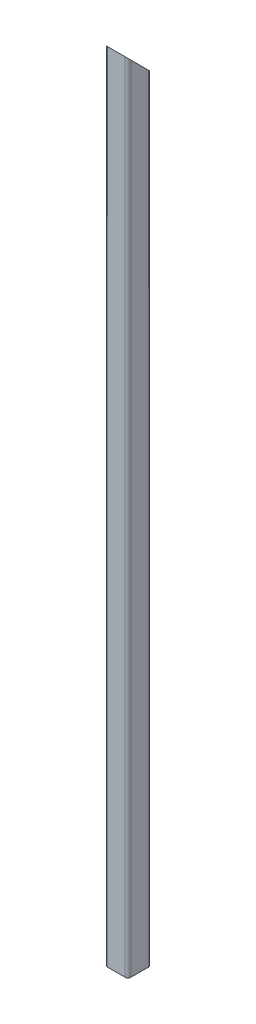
SolidWorks part; units mm, degrees
ref_plane "Front" through (0, 0, 0) normal (0, 0, 1) x (1, 0, 0)
ref_plane "Top" through (0, 0, 0) normal (0, 1, 0) x (1, 0, 0)
ref_plane "Right" through (0, 0, 0) normal (1, 0, 0) x (0, 0, -1)
sketch "草图1" plane through (0, 0, 0) normal (0, 1, 0) x (1, 0, 0)
  line L0 (-19, -7.2781) -> (19, -7.2781)
  line L1 (-19, -12.2781) -> (19, -12.2781)
  line L2 (-25, -6.2781) -> (-25, 31.7219)
  line L3 (-19, 37.7219) -> (19, 37.7219)
  line L4 (25, -6.2781) -> (25, 31.7219)
  line L5 (20, -6.2781) -> (20, 31.7219)
  line L6 (-19, 32.7219) -> (19, 32.7219)
  line L11 (-20, -6.2781) -> (-20, 31.7219)
  arc A0 (-19, -12.2781) -> (-25, -6.2781) centre (-19, -6.2781) cw
  arc A1 (19, -12.2781) -> (25, -6.2781) centre (19, -6.2781) ccw
  arc A2 (19, 37.7219) -> (25, 31.7219) centre (19, 31.7219) cw
  arc A3 (-25, 31.7219) -> (-19, 37.7219) centre (-19, 31.7219) cw
  arc A4 (19, -7.2781) -> (20, -6.2781) centre (19, -6.2781) ccw
  arc A5 (19, 32.7219) -> (20, 31.7219) centre (19, 31.7219) cw
  arc A6 (-20, 31.7219) -> (-19, 32.7219) centre (-19, 31.7219) cw
  arc A7 (-19, -7.2781) -> (-20, -6.2781) centre (-19, -6.2781) cw
  point P9 (25, -12.2781)
  point P12 (25, 37.7219)
  point P15 (-25, 37.7219)
  dimension "D3" = 6
  dimension "D1" = 50
  dimension "D2" = 50
  dimension "D4" = 5
extrude "凸台-拉伸1" add sketch "草图1" along normal blind 1775
sketch "草图2" plane through (25, 0, 0) normal (1, 0, 0) x (0, 0, -1)
  line L0 (-12.2781, 1775) -> (37.7219, 1775)
  line L1 (37.7219, 1775) -> (37.7219, 1725)
  line L2 (37.7219, 1775) -> (37.7219, 0) construction
  line L3 (37.7219, 1725) -> (-12.2781, 1775)
  dimension "D1" = 45
extrude "切除-拉伸1" cut sketch "草图2" against normal through all
sketch "草图3" plane through (0, 0, 0) normal (0, -1, 0) x (1, 0, 0)
  line L4 (-25, 6.2781) -> (-25, -31.7219)
  line L5 (-19, -37.7219) -> (19, -37.7219)
  line L6 (25, -31.7219) -> (25, 6.2781)
  line L7 (19, 12.2781) -> (-19, 12.2781)
  line L8 (-25, 6.2781) -> (-25, -31.7219)
  line L9 (-19, -37.7219) -> (19, -37.7219)
  line L10 (25, -31.7219) -> (25, 6.2781)
  line L11 (19, 12.2781) -> (-19, 12.2781)
  arc A4 (-19, 12.2781) -> (-25, 6.2781) centre (-19, 6.2781) ccw
  arc A5 (-25, -31.7219) -> (-19, -37.7219) centre (-19, -31.7219) ccw
  arc A6 (19, -37.7219) -> (25, -31.7219) centre (19, -31.7219) ccw
  arc A7 (25, 6.2781) -> (19, 12.2781) centre (19, 6.2781) ccw
  arc A8 (-19, 12.2781) -> (-25, 6.2781) centre (-19, 6.2781) ccw
  arc A9 (-25, -31.7219) -> (-19, -37.7219) centre (-19, -31.7219) ccw
  arc A10 (19, -37.7219) -> (25, -31.7219) centre (19, -31.7219) ccw
  arc A11 (25, 6.2781) -> (19, 12.2781) centre (19, 6.2781) ccw
  dimension "D1" = 0
extrude "凸台-拉伸2" add sketch "草图3" against normal blind 5
sketch "草图4" plane through (25, 0, 0) normal (1, 0, 0) x (0, 0, -1)
  line L0 (-6.2781, 0) -> (31.7219, 0) construction
  line L1 (-341.2655, 50) -> (254.9238, 50)
  line L2 (-341.2655, 50) -> (-341.2655, -272.9358)
  line L3 (-341.2655, -272.9358) -> (254.9238, -272.9358)
  line L4 (254.9238, 50) -> (254.9238, -272.9358)
  dimension "D1" = 50
extrude "切除-拉伸2" cut sketch "草图4" against normal through all
sketch "草图5" plane through (0, 50, 0) normal (0, -1, 0) x (1, 0, 0)
  line L4 (-25, 6.2781) -> (-25, -31.7219)
  line L5 (-19, -37.7219) -> (19, -37.7219)
  line L6 (25, -31.7219) -> (25, 6.2781)
  line L7 (19, 12.2781) -> (-19, 12.2781)
  line L8 (-25, 6.2781) -> (-25, -31.7219)
  line L9 (-19, -37.7219) -> (19, -37.7219)
  line L10 (25, -31.7219) -> (25, 6.2781)
  line L11 (19, 12.2781) -> (-19, 12.2781)
  arc A4 (-25, -31.7219) -> (-19, -37.7219) centre (-19, -31.7219) ccw
  arc A5 (19, -37.7219) -> (25, -31.7219) centre (19, -31.7219) ccw
  arc A6 (25, 6.2781) -> (19, 12.2781) centre (19, 6.2781) ccw
  arc A7 (-19, 12.2781) -> (-25, 6.2781) centre (-19, 6.2781) ccw
  arc A8 (-25, -31.7219) -> (-19, -37.7219) centre (-19, -31.7219) ccw
  arc A9 (19, -37.7219) -> (25, -31.7219) centre (19, -31.7219) ccw
  arc A10 (25, 6.2781) -> (19, 12.2781) centre (19, 6.2781) ccw
  arc A11 (-19, 12.2781) -> (-25, 6.2781) centre (-19, 6.2781) ccw
  dimension "D1" = 0
extrude "凸台-拉伸3" add sketch "草图5" against normal blind 10
